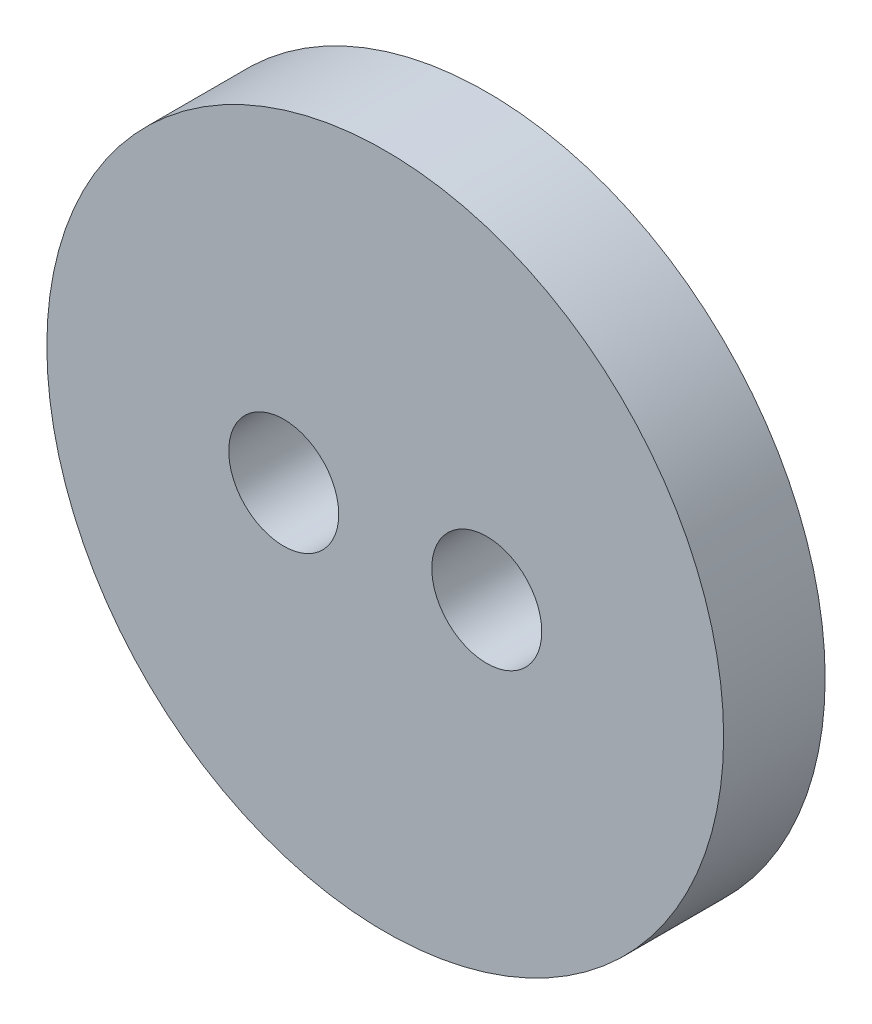
from build123d import *

# Parameters (mm, degrees)
SKETCH_1_R      = 20
SKETCH_1_R_2    = 3.25
EXTRUDE_1_DEPTH = 6


with BuildPart() as part:
    # 草图1 → 凸台-拉伸1 (new body)
    with BuildSketch(Plane.XY):
        Circle(SKETCH_1_R)
        with Locations((6, 0)):
            Circle(SKETCH_1_R_2, mode=Mode.SUBTRACT)
        with Locations((-6, 0)):
            Circle(SKETCH_1_R_2, mode=Mode.SUBTRACT)
    extrude(amount=EXTRUDE_1_DEPTH)


solid = part.part
